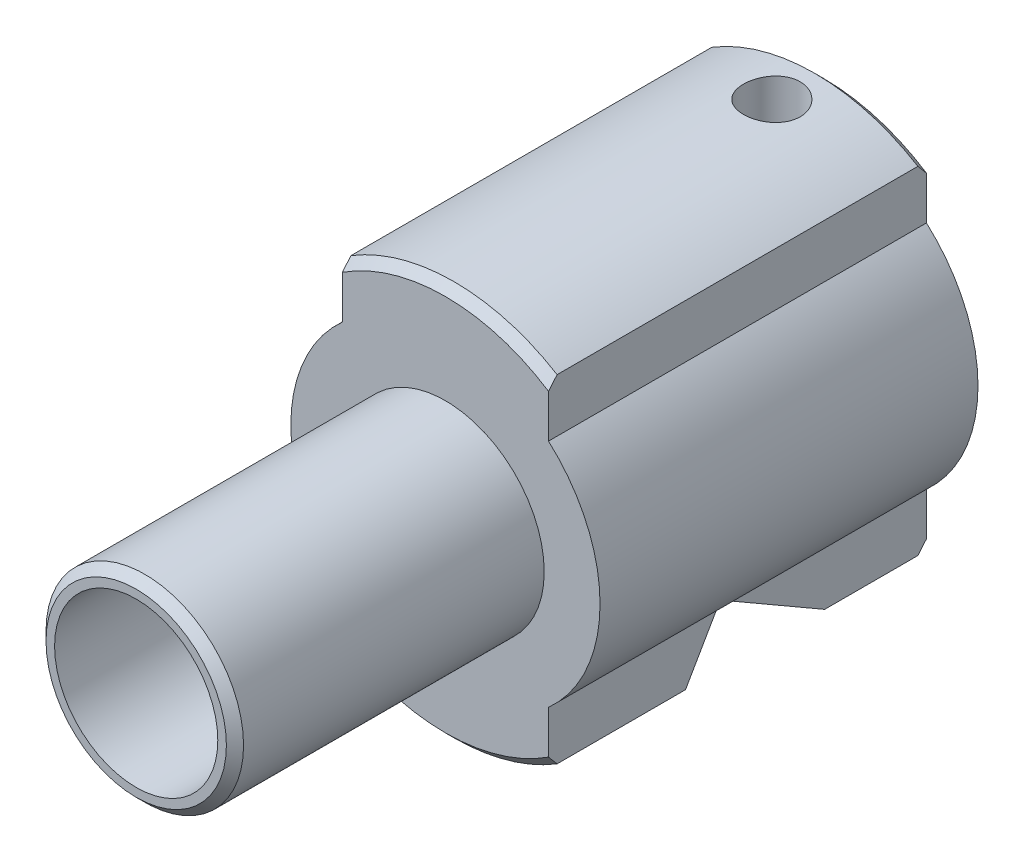
from build123d import *

# Parameters (mm, degrees)
SKETCH1_R                       = 11.5
SKETCH1_R_2                     = 4.75
BOSS_EXTRUDE1_DEPTH             = 22
SKETCH2_R                       = 5.75
SKETCH2_R_2                     = 4.75
BOSS_EXTRUDE2_DEPTH             = 18
SKETCH3_R                       = 6.5
CUT_EXTRUDE1_DEPTH              = 8
CHAMFER1_SIZE                   = 0.5
SKETCH12_W                      = 1.65
SKETCH12_H                      = 11.5
CUT_EXTRUDE4_DEPTH              = 44.179856468
CUT_EXTRUDE4_DEPTH_BACK         = 44.179856468
F_1_2_1_2_DIAMETER_HOLE1_REACH  = 40.711
F_1_2_1_2_DIAMETER_HOLE1_BORE_R = 0.6
M3_TAPPED_HOLE2_D               = 2.5
M3_TAPPED_HOLE2_DEPTH           = 4.5
M3_TAPPED_HOLE2_TIP             = 0.751075774
CHAMFER2_SIZE                   = 0.3
CHAMFER2_SIZE2                  = 8
CUT_EXTRUDE5_DEPTH              = 44.179856561
CHAMFER3_SIZE                   = 0.5


with BuildPart() as part:
    # Sketch1 → Boss-Extrude1 (new body)
    with BuildSketch(Plane.XY):
        Circle(SKETCH1_R)
        Circle(SKETCH1_R_2, mode=Mode.SUBTRACT)
    extrude(amount=BOSS_EXTRUDE1_DEPTH)

    # Sketch2 → Boss-Extrude2 (add)
    with BuildSketch(Plane.XY.offset(22)):
        Circle(SKETCH2_R)
        Circle(SKETCH2_R_2, mode=Mode.SUBTRACT)
    extrude(amount=BOSS_EXTRUDE2_DEPTH)

    # Sketch3 → Cut-Extrude1 (cut)
    with BuildSketch(Plane(origin=(0, 0, 0), x_dir=(-1, 0, 0), z_dir=(0, 0, -1))):
        Circle(SKETCH3_R)
    extrude(amount=-CUT_EXTRUDE1_DEPTH, mode=Mode.SUBTRACT)

    # Chamfer1
    chamfer1_edges = [part.edges().sort_by_distance(p)[0] for p in [
        (-11.5, 0, 0),
        (-11.5, 0, 22),
    ]]
    chamfer(chamfer1_edges, length=CHAMFER1_SIZE)

    # Sketch12 → M4 Tapped Hole3 (revolve, cut)
    with BuildSketch(Plane(origin=(0, 0, 3), x_dir=(0, 0, -1), z_dir=(1, 0, 0))):
        with Locations((0.825, 5.75)):
            Rectangle(SKETCH12_W, SKETCH12_H)
    revolve(axis=Axis((0, -6.35, 3), (0, 1, 0)), mode=Mode.SUBTRACT)

    # Sketch14 → Cut-Extrude4 (cut, two sides: drawn at the far end of the back side and taken through both)
    with BuildSketch(Plane(origin=(0, 0, 0), x_dir=(0, 0, -1), z_dir=(1, 0, 0)).offset(-CUT_EXTRUDE4_DEPTH_BACK)):
        Polygon((-15, -11.5), (-12, -6.303847577), (-3, -11.5), align=None)
    extrude(amount=CUT_EXTRUDE4_DEPTH + CUT_EXTRUDE4_DEPTH_BACK, mode=Mode.SUBTRACT)

    # Ø1.2 (1.2) Diameter Hole1 bore → Ø1.2 (1.2) Diameter Hole1 (cut, up to next)
    with BuildSketch(Plane(origin=(0, 3.620190528, 6.270353928), x_dir=(-1, 0, 0), z_dir=(0, -0.5000000000000001, -0.8660254037844386)), mode=Mode.PRIVATE) as f_1_2_1_2_diameter_hole1_sk1:
        with Locations((0, -14.459292144)):
            Circle(F_1_2_1_2_DIAMETER_HOLE1_BORE_R)
    f_1_2_1_2_diameter_hole1_tool1 = extrude(f_1_2_1_2_diameter_hole1_sk1.sketch, amount=-F_1_2_1_2_DIAMETER_HOLE1_REACH, mode=Mode.PRIVATE) & part.part
    add(f_1_2_1_2_diameter_hole1_tool1.solids().sort_by_distance((0, -8.901924, 13.5))[0], mode=Mode.SUBTRACT)

    # M3 Tapped Hole2
    with Locations(Plane(origin=(0, 3.620190528, 6.270353928), x_dir=(-1, 0, 0), z_dir=(0, -0.5000000000000001, -0.8660254037844386))):
        with Locations((0, -14.459292144)):
            Hole(M3_TAPPED_HOLE2_D / 2, depth=M3_TAPPED_HOLE2_DEPTH)
            with Locations((0, 0, -(M3_TAPPED_HOLE2_DEPTH + M3_TAPPED_HOLE2_TIP / 2))):  # 118° drill point
                Cone(0, M3_TAPPED_HOLE2_D / 2, M3_TAPPED_HOLE2_TIP, mode=Mode.SUBTRACT)

    # Chamfer2
    chamfer2_edges = [part.edges().sort_by_distance(p)[0] for p in [
        (-4.75, 0, 8),
    ]]
    chamfer2_side = [part.faces().sort_by_distance(p)[0] for p in [
        (6.316152237, 0, 8),
    ]]
    chamfer(chamfer2_edges, length=CHAMFER2_SIZE, length2=CHAMFER2_SIZE2, reference=chamfer2_side[0])

    # Sketch19 → Cut-Extrude5 (cut, through all)
    with BuildSketch(Plane(origin=(0, 0, 0), x_dir=(-1, 0, 0), z_dir=(0, 0, -1))):
        with BuildLine():
            Line((-6, 9.810708435), (-6, 6.708203932))
            ThreePointArc((-6, 6.708203932), (-9, 0), (-6, -6.708203932))
            Line((-6, -6.708203932), (-6, -9.810708435))
            ThreePointArc((-6, -9.810708435), (-11.5, 0), (-6, 9.810708435))
        make_face()
        with BuildLine():
            Line((6, 9.810708435), (6, 6.708203932))
            ThreePointArc((6, 6.708203932), (9, 0), (6, -6.708203932))
            Line((6, -6.708203932), (6, -9.810708435))
            ThreePointArc((6, -9.810708435), (11.5, 0), (6, 9.810708435))
        make_face()
    extrude(amount=-CUT_EXTRUDE5_DEPTH, mode=Mode.SUBTRACT)

    # Chamfer3
    chamfer3_edges = [part.edges().sort_by_distance(p)[0] for p in [
        (-5.75, 0, 40),
        (6.5, 0, 0),
    ]]
    chamfer(chamfer3_edges, length=CHAMFER3_SIZE)


solid = part.part
